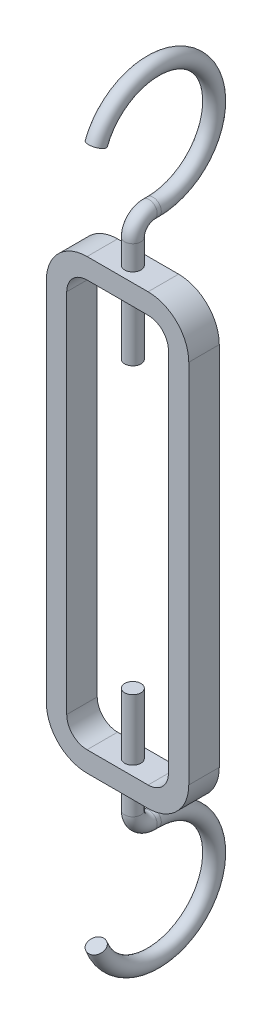
from build123d import *

# Parameters (mm, degrees)
EXTRUDE_1_DEPTH = 7.5
SKETCH_6_R      = 4
SKETCH_7_R      = 4
EXTRUDE_2_DEPTH = 30


with BuildPart() as part:
    # 草图4 → 凸台-拉伸1 (new, symmetric)
    with BuildSketch(Plane.XY):
        with BuildLine():
            Line((-15, 110), (15, 110))
            ThreePointArc((15, 110), (29.142135624, 104.142135624), (35, 90))
            Line((35, 90), (35, -90))
            ThreePointArc((35, -90), (29.142135624, -104.142135624), (15, -110))
            Line((15, -110), (-15, -110))
            ThreePointArc((-15, -110), (-29.142135624, -104.142135624), (-35, -90))
            Line((-35, -90), (-35, 90))
            ThreePointArc((-35, 90), (-29.142135624, 104.142135624), (-15, 110))
        make_face()
        with BuildLine():
            Line((-15, -100), (15, -100))
            ThreePointArc((15, -100), (22.071067812, -97.071067812), (25, -90))
            Line((25, -90), (25, 90))
            ThreePointArc((25, 90), (22.071067812, 97.071067812), (15, 100))
            Line((15, 100), (-15, 100))
            ThreePointArc((-15, 100), (-22.071067812, 97.071067812), (-25, 90))
            Line((-25, 90), (-25, -90))
            ThreePointArc((-25, -90), (-22.071067812, -97.071067812), (-15, -100))
        make_face(mode=Mode.SUBTRACT)
    extrude(amount=EXTRUDE_1_DEPTH, both=True)

    # 扫描1: sweep along a path in 草图5
    with BuildLine(Plane(origin=(0, 0, 0), x_dir=(0, 0, -1), z_dir=(1, 0, 0))) as sweep_1_path:
        Line((0, 110), (0, 122))
        ThreePointArc((0, 122), (2.343145751, 127.656854249), (8, 130))
        Line((8, 130), (10, 130))
        ThreePointArc((10, 130), (34.729636961, 176.983670268), (-18, 170.770329614))
    # 草图6 → 扫描1 (sweep)
    with BuildSketch(Plane(origin=(0, 110, 0), x_dir=(1, 0, 0), z_dir=(0, 1, 0))):
        Circle(SKETCH_6_R)
    sweep_1 = sweep(path=sweep_1_path.line)

    # 草图7 → 凸台-拉伸2 (add)
    with BuildSketch(Plane.XZ.offset(-100)):
        with Locations(Location((0, 0, 0), (0, 0, 90))):
            Circle(SKETCH_7_R)
    extrude_2 = extrude(amount=EXTRUDE_2_DEPTH)

    # 镜向1: 扫描1, 凸台-拉伸2 across plane
    add(sweep_1.mirror(Plane.ZX))
    add(extrude_2.mirror(Plane.ZX))


solid = part.part
